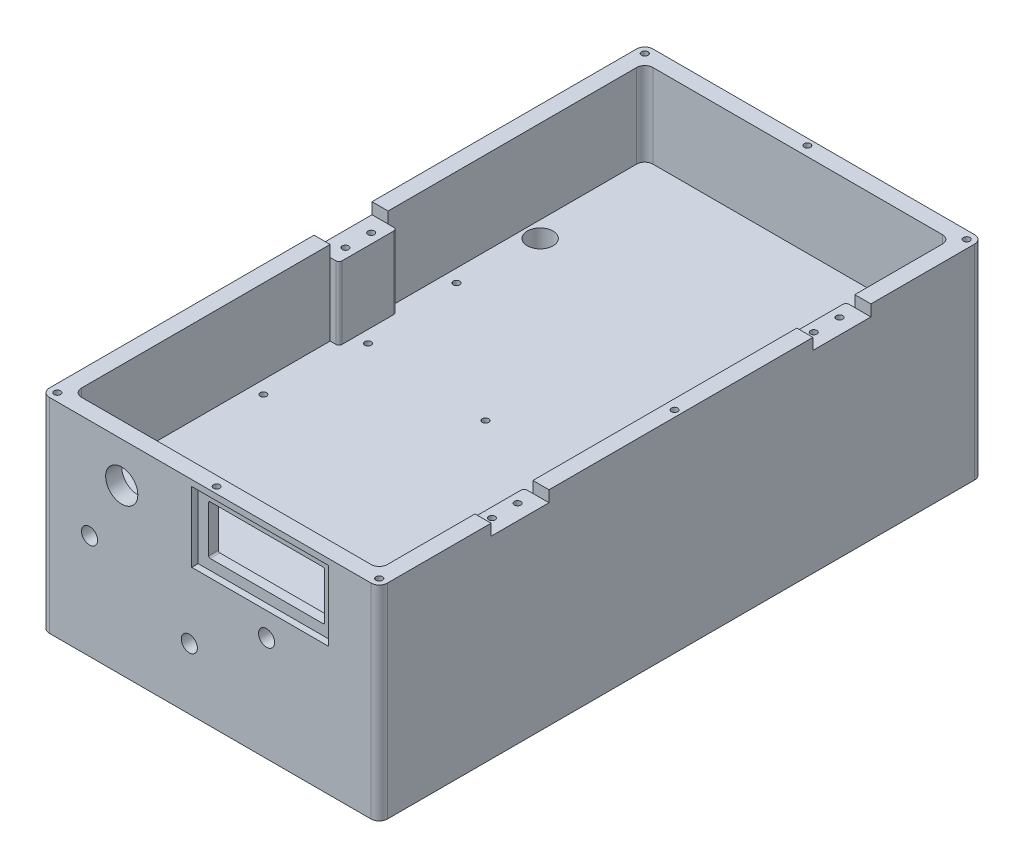
SolidWorks part; units mm, degrees
ref_plane "Front Plane" through (0, 0, 0) normal (0, 0, 1) x (1, 0, 0)
ref_plane "Top Plane" through (0, 0, 0) normal (0, 1, 0) x (1, 0, 0)
ref_plane "Right Plane" through (0, 0, 0) normal (1, 0, 0) x (0, 0, -1)
sketch "Sketch1" plane through (0, 0, 0) normal (0, 1, 0) x (1, 0, 0)
  line L1 (0, 0) -> (200, 0)
  line L2 (0, 0) -> (0, 400)
  line L3 (0, 400) -> (200, 400)
  line L4 (200, 0) -> (200, 400)
extrude "Boss-Extrude1" add sketch "Sketch1" along normal blind 25
sketch "Sketch2" plane through (0, 0, 0) normal (0, -1, 0) x (1, 0, 0)
  line L0 (0, -400) -> (0, 0) construction
  line L1 (37.7823, -177.17) -> (65.6061, -192.9762) construction
  line L2 (200, -400) -> (0, -400) construction
  line L3 (21.9762, -204.9939) -> (8.0642, -197.0908) construction
  circle A0 centre (70, -320) radius 1
  circle A1 centre (68.3, -276.5) radius 1
  circle A2 centre (66, -139.3) radius 1
  circle A3 centre (50, -320) radius 1
  circle A4 centre (50, -300) radius 1
  circle A5 centre (70, -300) radius 1
  circle A6 centre (48.3, -276.5) radius 1
  circle A7 centre (46, -139.3) radius 1
  circle A8 centre (48.3, -256.5) radius 1
  circle A9 centre (46, -119.3) radius 1
  circle A10 centre (68.3, -256.5) radius 1
  circle A11 centre (66, -119.3) radius 1
  circle A12 centre (49.8, -220.8) radius 1.5
  circle A13 centre (65.6061, -192.9762) radius 1.5
  circle A14 centre (37.7823, -177.17) radius 1.5
  circle A15 centre (21.9762, -204.9939) radius 1.5
  circle A16 centre (51.6942, -185.0731) radius 1.5
  circle A17 centre (8.0642, -197.0908) radius 1.5
  dimension "D1" = 70
  dimension "D2" = 80
  dimension "D3" = 43.5
  dimension "D4" = 1.7
  dimension "D5" = 180.7
  dimension "D6" = 4
  dimension "D11" = 99.2
  dimension "D12" = 20.2
  dimension "D7" = 2
  dimension "D8" = 2
  dimension "D9" = 2
  dimension "D10" = 2
  dimension "D13" = 2
  dimension "D14" = 2
extrude "Cut-Extrude1" cut sketch "Sketch2" against normal blind 5
sketch "Sketch3" plane through (0, 0, 0) normal (0, -1, 0) x (1, 0, 0)
  line L0 (66, -119.3) -> (46, -139.3) construction
  line L1 (56, -129.3) -> (57.9085, -144.8434) construction
  line L2 (0, -400) -> (0, 0) construction
  line L3 (57.9085, -144.8434) -> (97.891, -305.2047) construction
  line L4 (97.891, -305.2047) -> (64.0384, -102.9093) construction
  line L5 (64.0384, -102.9093) -> (134.2678, -301.231) construction
  line L6 (134.2678, -301.231) -> (118.7891, -68.1883) construction
  line L7 (118.7891, -68.1883) -> (118.7891, -348.1883) construction
  line L8 (68.3, -256.5) -> (48.3, -276.5) construction
  line L9 (58.3, -266.5) -> (60.0513, -252.2371) construction
  line L10 (60.0513, -252.2371) -> (96.3395, -106.6928) construction
  line L11 (96.3395, -106.6928) -> (82.5516, -353.3076) construction
  line L12 (82.5516, -353.3076) -> (82.5516, -73.3076) construction
  dimension "D1" = 7
  dimension "D2" = 14
  dimension "D3" = 4.5
  dimension "D4" = 10
  dimension "D5" = 15.7
  dimension "D6" = 7
  dimension "D7" = 14
  dimension "D8" = 10.8
sketch "Sketch4" plane through (0, 0, 0) normal (0, -1, 0) x (1, 0, 0)
  line L0 (97.891, -305.2047) -> (101.3054, -321.6196) construction
  line L1 (97.891, -305.2047) -> (64.0384, -102.9093) construction
  line L2 (64.0384, -102.9093) -> (59.8238, -86.6126) construction
  line L3 (64.0384, -102.9093) -> (134.2678, -301.231) construction
  line L5 (134.2678, -301.231) -> (137.9976, -319.3208) construction
  line L6 (134.2678, -301.231) -> (118.7891, -68.1883) construction
  line L7 (118.7891, -68.1883) -> (118.4009, -56.4845) construction
  line L8 (118.7891, -68.1883) -> (118.7891, -348.1883) construction
  line L9 (96.3395, -106.6928) -> (98.8592, -90.0322) construction
  line L10 (96.3395, -106.6928) -> (82.5516, -353.3076) construction
  line L11 (82.5516, -353.3076) -> (82.0812, -370.1511) construction
  line L14 (82.5516, -353.3076) -> (82.5516, -73.3076) construction
  line L16 (118.7891, -348.1883) -> (118.7891, -367.68) construction
  line L17 (82.5516, -73.3076) -> (82.5516, -58.9376) construction
  dimension "D2" = 5
  dimension "D3" = 7.85
  dimension "D4" = 1.9
  dimension "D5" = 5.4
  dimension "D6" = 1.6
  dimension "D1" = 2.25
sketch "Sketch6" plane through (0, 0, 0) normal (0, -1, 0) x (1, 0, 0)
  circle A0 centre (82, -370) radius 2
  circle A1 centre (70, -320) radius 1 construction
  circle A2 centre (59.7, -86.5) radius 2
  circle A4 centre (119.5, -370) radius 2
  circle A5 centre (82, -56.5) radius 2
  circle A6 centre (101.2, -321.7) radius 2
  circle A7 centre (138.2, -321.7) radius 2
  circle A8 centre (119, -56.5) radius 2
  circle A9 centre (99, -90) radius 2
  dimension "D1" = 50
  dimension "D2" = 12
  dimension "D3" = 37.5
  dimension "D4" = 313.5
  dimension "D5" = 12
  dimension "D6" = 48.3
  dimension "D7" = 19.2
  dimension "D8" = 37
  dimension "D9" = 37
  dimension "D10" = 17
  dimension "D11" = 33.5
  dimension "D12" = 22.3
  dimension "D13" = 30
sketch "Sketch7" plane through (0, 0, 0) normal (0, -1, 0) x (1, 0, 0)
  line L1 (200, 0) -> (-100, 0) construction
  line L2 (200, 0) -> (200, -530) construction
  line L3 (200, -530) -> (-100, -530) construction
  line L4 (-100, 0) -> (-100, -530) construction
sketch "Sketch9" plane through (0, 0, 0) normal (0, -1, 0) x (1, 0, 0)
  line L0 (75, -330) -> (90, -330)
  line L1 (50, -99) -> (200, -99)
  line L3 (110, 0) -> (200, 0)
  line L4 (200, -99) -> (200, 0)
  line L5 (200, 0) -> (200, -530) construction
  line L6 (200, -315) -> (90, -315)
  line L7 (200, -315) -> (200, -400)
  line L8 (200, -400) -> (75, -400)
  line L10 (200, -400) -> (0, -400) construction
  line L12 (75, -400) -> (40, -400)
  line L13 (40, -400) -> (40, -330)
  line L14 (40, -330) -> (75, -330)
  line L15 (90, -330) -> (90, -315)
  line L16 (50, -99) -> (50, -79)
  line L17 (50, -79) -> (100, -79)
  line L19 (100, -79) -> (110, -79)
  line L20 (110, -79) -> (110, 0)
  dimension "D1" = 85
  dimension "D3" = 35
extrude "Boss-Extrude2" add sketch "Sketch9" along normal blind 12
sketch "Sketch10" plane through (0, -12, 0) normal (0, -1, 0) x (1, 0, 0)
  circle A0 centre (82, -56.5) radius 2
  circle A1 centre (119, -56.5) radius 2
  circle A2 centre (59.7, -86.5) radius 2
  circle A3 centre (99, -90) radius 2
  circle A4 centre (138.2, -321.7) radius 2
  circle A5 centre (119.5, -370) radius 2
  circle A6 centre (101.2, -321.7) radius 2
  circle A7 centre (82, -370) radius 2
extrude "Cut-Extrude2" cut sketch "Sketch10" against normal blind 5
sketch "Sketch11" plane through (0, 25, 0) normal (0, 1, 0) x (1, 0, 0)
  line L0 (200, 400) -> (0, 400) construction
  line L1 (200, 0) -> (200, 530) construction
  line L2 (161, 200) -> (155.25, 200) construction
  line L3 (155.25, 200) -> (155.25, 273.7112) construction
  circle A0 centre (161, 200) radius 2
  circle A7 centre (91, 200) radius 2
  circle A8 centre (91, 42) radius 2
  circle A9 centre (161, 42) radius 2
  dimension "D1" = 2
  dimension "D3" = 200
  dimension "D4" = 39
  dimension "D5" = 5.75
  dimension "D2" = 2
extrude "Cut-Extrude3" cut sketch "Sketch11" against normal blind 5
sketch "Sketch13" plane through (0, 0, 0) normal (0, -1, 0) x (1, 0, 0)
  line L0 (155.25, -235) -> (155.25, -266) construction
  line L1 (165.75, -235) -> (144.75, -235)
  line L2 (165.75, -235) -> (165.75, -266)
  line L4 (144.75, -235) -> (144.75, -266)
  line L5 (200, 0) -> (200, -530) construction
  line L6 (200, 0) -> (-100, 0) construction
  line L7 (165.75, -266) -> (155.25, -266)
  line L8 (155.25, -266) -> (144.75, -266)
  dimension "D1" = 44.75
  dimension "D2" = 235
extrude "Cut-Extrude4" cut sketch "Sketch13" against normal blind 157
sketch "Sketch14" plane through (0, -12, 0) normal (0, -1, 0) x (1, 0, 0)
  line L0 (200, 0) -> (200, -530) construction
  line L1 (40, -400) -> (200, -400) construction
  line L2 (155.25, -330) -> (165.4111, -340.1611) construction
  line L3 (50, -320) -> (70, -320) construction
  line L4 (60, -320) -> (60, -330) construction
  line L5 (155.25, -330) -> (60, -330) construction
  line L6 (60, -330) -> (49.8389, -340.1611) construction
  circle A0 centre (155.25, -330) radius 2 construction
  circle A1 centre (165.4111, -340.1611) radius 2
  circle A2 centre (49.8389, -340.1611) radius 2
  dimension "D1" = 44.75
  dimension "D2" = 70
  dimension "D3" = 45
extrude "Cut-Extrude5" cut sketch "Sketch14" against normal blind 5
sketch "Sketch15" plane through (0, 0, 0) normal (0, 0, 1) x (1, 0, 0)
  line L0 (0, 25) -> (200, 25) construction
  line L1 (200, 25) -> (200, -12) construction
  circle A1 centre (130, 15) radius 3.5
  dimension "D1" = 10
  dimension "D3" = 70
extrude "Cut-Extrude6" cut sketch "Sketch15" against normal blind 175
sketch "Sketch16" plane through (0, 0, 0) normal (0, -1, 0) x (1, 0, 0)
  line L0 (200, 0) -> (200, -530) construction
  line L1 (200, 0) -> (-100, 0) construction
  line L2 (0, -400) -> (0, 0) construction
  circle A0 centre (130, -170) radius 3.5
  circle A1 centre (20, -265) radius 3.5
  dimension "D1" = 70
  dimension "D2" = 170
  dimension "D3" = 265
  dimension "D4" = 20
extrude "Cut-Extrude7" cut sketch "Sketch16" against normal blind 20
sketch "Sketch17" plane through (0, 0, 0) normal (0, 0, 1) x (1, 0, 0)
  line L0 (0, 25) -> (200, 25) construction
  line L1 (0, 25) -> (0, 0) construction
  circle A0 centre (20, 15) radius 3.5
  dimension "D1" = 10
  dimension "D2" = 20
extrude "Cut-Extrude8" cut sketch "Sketch17" against normal blind 270
sketch "Sketch18" plane through (0, 0, 0) normal (0, -1, 0) x (1, 0, 0)
  circle A0 centre (130, -170) radius 4
  circle A1 centre (20, -265) radius 4
extrude "Cut-Extrude9" cut sketch "Sketch18" against normal blind 7
sketch "Sketch19" plane through (0, 0, 0) normal (0, -1, 0) x (1, 0, 0)
  line L0 (165.75, -250.5) -> (181.25, -250.5) construction
  line L1 (165.75, -266) -> (165.75, -235) construction
  line L2 (144.75, -250.5) -> (131.25, -250.5) construction
  line L3 (144.75, -235) -> (144.75, -266) construction
  circle A0 centre (181.25, -250.5) radius 2
  circle A1 centre (131.25, -250.5) radius 2
extrude "Cut-Extrude10" cut sketch "Sketch19" against normal blind 5
sketch "Sketch20" plane through (0, -12, 0) normal (0, -1, 0) x (1, 0, 0)
  line L1 (200, 0) -> (0, 0)
  line L2 (200, 0) -> (200, -35)
  line L3 (200, -35) -> (0, -35)
  line L4 (0, 0) -> (0, -35)
extrude "Cut-Extrude11" cut sketch "Sketch20" against normal blind 98
sketch "Sketch21" plane through (0, 0, 0) normal (0, -1, 0) x (1, 0, 0)
  line L0 (82, -56.5) -> (72, -56.5) construction
  line L1 (72, -56.5) -> (72, -46.5) construction
  circle A0 centre (72, -46.5) radius 1
  circle A1 centre (92, -46.5) radius 1
  circle A2 centre (92, -66.5) radius 1
  circle A3 centre (72, -66.5) radius 1
  dimension "D1" = 2
  dimension "D2" = 2
extrude "Cut-Extrude12" cut sketch "Sketch21" against normal blind 5
sketch "Sketch22" plane through (0, -12, 0) normal (0, -1, 0) x (1, 0, 0)
  line L0 (200, 0) -> (200, -530) construction
  line L1 (40, -400) -> (200, -400) construction
  line L2 (0, -400) -> (0, -35) construction
  line L3 (0, -35) -> (110, -35) construction
  circle A0 centre (160, -370) radius 3.25
  circle A1 centre (23, -370) radius 3.25
  circle A2 centre (54, -60) radius 3.25
  dimension "D1" = 40
  dimension "D2" = 30
  dimension "D3" = 137
  dimension "D4" = 54
  dimension "D5" = 25
extrude "Cut-Extrude13" [suppressed] cut sketch "Sketch22" against normal blind 84
sketch "Sketch23" [suppressed] plane through (0, 0, 0) normal (0, -1, 0) x (1, 0, 0)
  circle A0 centre (54, -60) radius 6.25
  circle A1 centre (23, -370) radius 6.25
extrude "Cut-Extrude14" [suppressed] cut sketch "Sketch23" against normal blind 22
sketch "Sketch24" [suppressed] plane through (0, -12, 0) normal (0, -1, 0) x (1, 0, 0)
  circle A0 centre (160, -370) radius 6.25
extrude "Cut-Extrude15" [suppressed] cut sketch "Sketch24" against normal blind 34
sketch "Sketch27" plane through (0, 0, -35) normal (0, 0, 1) x (1, 0, 0)
  line L1 (0, 25) -> (200, 25)
  line L2 (0, 25) -> (0, -50)
  line L3 (0, -50) -> (200, -50)
  line L4 (200, 25) -> (200, -50)
  circle A1 centre (130, 15) radius 3.5
  circle A2 centre (20, 15) radius 3.5
extrude "Boss-Extrude3" add sketch "Sketch27" along normal blind 10
sketch "Sketch28" plane through (0, 0, -25) normal (0, 0, 1) x (1, 0, 0)
  line L0 (0, 25) -> (0, -50) construction
  line L1 (200, 25) -> (0, 25) construction
  circle A0 centre (82, -12) radius 5
  dimension "D1" = 82
  dimension "D2" = 37
extrude "Cut-Extrude16" cut sketch "Sketch28" against normal blind 10
sketch "Sketch29" plane through (0, 0, 0) normal (0, -1, 0) x (1, 0, 0)
  circle A2 centre (103, -59.5) radius 1.5
  circle A3 centre (92, -66.5) radius 1 construction
  circle A4 centre (103, -63.5) radius 1.5
  dimension "D1" = 4
  dimension "D2" = 11
  dimension "D3" = 7
extrude "Cut-Extrude17" cut sketch "Sketch29" against normal blind 5
sketch "Sketch30" plane through (0, 0, 0) normal (-1, 0, 0) x (0, 0, 1)
  line L1 (-25, 25) -> (-400, 25)
  line L2 (-25, 25) -> (-25, -50)
  line L3 (-25, -50) -> (-400, -50)
  line L4 (-400, 25) -> (-400, -50)
extrude "Boss-Extrude4" add sketch "Sketch30" along normal blind 10
sketch "Sketch31" plane through (0, 0, -400) normal (0, 0, -1) x (-1, 0, 0)
  line L1 (10, -50) -> (-200, -50)
  line L2 (10, -50) -> (10, 25)
  line L3 (10, 25) -> (-200, 25)
  line L4 (-200, -50) -> (-200, 25)
extrude "Boss-Extrude5" add sketch "Sketch31" against normal blind 10
sketch "Sketch32" plane through (200, 0, 0) normal (1, 0, 0) x (0, 0, -1)
  line L1 (400, -50) -> (25, -50)
  line L2 (400, -50) -> (400, 25)
  line L3 (400, 25) -> (25, 25)
  line L4 (25, -50) -> (25, 25)
extrude "Boss-Extrude6" add sketch "Sketch32" against normal blind 10
sketch "Sketch33" plane through (0, -12, 0) normal (0, -1, 0) x (1, 0, 0)
  line L0 (190, -390) -> (0, -390) construction
  line L1 (40, -330) -> (40, -390) construction
  circle A0 centre (95, -341) radius 1.5
  circle A1 centre (140, -341) radius 1.5
  dimension "D1" = 49
  dimension "D2" = 55
  dimension "D3" = 45
extrude "Cut-Extrude18" cut sketch "Sketch33" against normal blind 5
sketch "Sketch34" plane through (0, 25, 0) normal (0, 1, 0) x (1, 0, 0)
  line L1 (200, 400) -> (-10, 400)
  line L2 (200, 400) -> (200, 25)
  line L3 (200, 25) -> (-10, 25)
  line L4 (-10, 400) -> (-10, 25)
  line L5 (190, 390) -> (190, 35)
  line L6 (190, 35) -> (0, 35)
  line L7 (0, 35) -> (0, 390)
  line L8 (0, 390) -> (190, 390)
extrude "Boss-Extrude7" add sketch "Sketch34" along normal blind 52
sketch "Sketch35" plane through (0, 0, -25) normal (0, 0, 1) x (1, 0, 0)
  line L0 (-10, -50) -> (200, -50) construction
  line L1 (167, 70) -> (87, 70)
  line L2 (167, 70) -> (167, 40)
  line L3 (167, 40) -> (87, 40)
  line L4 (87, 70) -> (87, 40)
  line L5 (200, -50) -> (200, 77) construction
  dimension "D1" = 30
  dimension "D2" = 80
  dimension "D3" = 90
  dimension "D4" = 33
extrude "Cut-Extrude19" cut sketch "Sketch35" against normal blind 35
sketch "Sketch36" plane through (0, -50, 0) normal (0, -1, 0) x (1, 0, 0)
  line L0 (0, -390) -> (0, -35) construction
  line L1 (-3, -391) -> (-1, -391)
  line L2 (-3, -391) -> (-3, -34)
  line L3 (-3, -34) -> (-1, -34)
  line L4 (-1, -391) -> (-1, -34)
  line L5 (190, -390) -> (0, -390) construction
  line L6 (0, -35) -> (190, -35) construction
  line L7 (95, -400) -> (95, -25) construction
  line L8 (-10, -400) -> (200, -400) construction
  line L9 (-10, -25) -> (200, -25) construction
  line L10 (191, -391) -> (191, -34)
  line L11 (193, -34) -> (191, -34)
  line L12 (193, -391) -> (193, -34)
  line L13 (193, -391) -> (191, -391)
  dimension "D1" = 2
  dimension "D2" = 1
  dimension "D3" = 1
  dimension "D4" = 1
extrude "Cut-Extrude20" cut sketch "Sketch36" against normal blind 1.5
sketch "Sketch37" plane through (0, -50, 0) normal (0, -1, 0) x (1, 0, 0)
  line L1 (-3, -391) -> (193, -391)
  line L2 (-3, -391) -> (-3, -393)
  line L3 (-3, -393) -> (193, -393)
  line L4 (193, -391) -> (193, -393)
  line L5 (-3, -34) -> (193, -34)
  line L6 (-3, -34) -> (-3, -32)
  line L7 (-3, -32) -> (193, -32)
  line L8 (193, -34) -> (193, -32)
extrude "Cut-Extrude21" cut sketch "Sketch37" against normal blind 1.5
sketch "Sketch38" plane through (0, -50, 0) normal (0, -1, 0) x (1, 0, 0)
  line L0 (-10, -25) -> (200, -25) construction
  line L1 (193, -393) -> (193, -32) construction
  line L4 (95, -400) -> (95, -25) construction
  line L5 (-10, -400) -> (200, -400) construction
  line L6 (-10, -212.5) -> (200, -212.5) construction
  line L7 (-10, -400) -> (-10, -25) construction
  line L8 (200, 0) -> (200, -530) construction
  circle A1 centre (195, -30) radius 2
  circle A5 centre (95, -396) radius 2
  circle A6 centre (95, -29) radius 2
  circle A7 centre (-6, -212.5) radius 2
  circle A8 centre (196, -212.5) radius 2
  circle A9 centre (-5, -30) radius 2
  circle A10 centre (-5, -395) radius 2
  circle A11 centre (195, -395) radius 2
  dimension "D1" = 5
  dimension "D2" = 2
  dimension "D3" = 2
  dimension "D4" = 2
extrude "Cut-Extrude22" cut sketch "Sketch38" against normal blind 5
fillet "Fillet1" radius 5 4 edges at (200, 13.5, -25) (-10, 13.5, -25) (200, 13.5, -400) (-10, 13.5, -400)
fillet "Fillet4" radius 5 4 edges at (190, -31, -35) (0, -25, -35) (0, -25, -390) (190, -31, -390)
fillet "Fillet5" radius 5 8 edges at (-1, -49.25, -34) (-3, -49.25, -32) (191, -49.25, -34) (193, -49.25, -32) (193, -49.25, -393) (191, -49.25, -391) (-1, -49.25, -391) (-3, -49.25, -393)
fillet "Fillet6" radius 5 4 edges at (0, 51, -35) (190, 51, -35) (0, 51, -390) (190, 51, -390)
sketch "Sketch41" plane through (0, 0, -400) normal (0, 0, -1) x (-1, 0, 0)
  line L0 (-200, -50) -> (-200, 77) construction
  line L1 (5, -50) -> (-195, -50) construction
  circle A0 centre (-119.5, -24.7) radius 5
  dimension "D1" = 80.5
  dimension "D2" = 25.3
extrude "Cut-Extrude23" cut sketch "Sketch41" against normal blind 28
sketch "Sketch42" plane through (0, -12, 0) normal (0, -1, 0) x (1, 0, 0)
  line L0 (-5, -400) -> (195, -400) construction
  line L1 (200, 0) -> (200, -530) construction
  circle A0 centre (155, -375) radius 2
  dimension "D1" = 25
  dimension "D2" = 45
extrude "Cut-Extrude24" cut sketch "Sketch42" against normal blind 5
sketch "Sketch43" plane through (0, 0, 0) normal (0, -1, 0) x (1, 0, 0)
  line L0 (-10, -395) -> (-10, -30) construction
  line L1 (-5, -400) -> (195, -400) construction
  circle A0 centre (10, -385) radius 2
  circle A1 centre (10, -364) radius 2
  dimension "D1" = 21
  dimension "D2" = 20
  dimension "D3" = 15
extrude "Cut-Extrude25" cut sketch "Sketch43" against normal blind 5
sketch "Sketch44" plane through (0, 0, 0) normal (0, -1, 0) x (1, 0, 0)
  line L0 (-5, -400) -> (195, -400) construction
  line L1 (-10, -395) -> (-10, -30) construction
  circle A0 centre (10, -315) radius 8
  dimension "D1" = 85
  dimension "D2" = 20
extrude "Cut-Extrude26" cut sketch "Sketch44" against normal blind 59
sketch "Sketch45" plane through (0, 25, 0) normal (0, 1, 0) x (1, 0, 0)
  line L0 (0, 385) -> (0, 40) construction
  circle A0 centre (8, 265) radius 2
  circle A1 centre (8, 205) radius 2 construction
  circle A2 centre (8, 145) radius 2
  circle A3 centre (8, 85) radius 2
  circle A4 centre (13, 205) radius 2
  dimension "D1" = 8
  dimension "D2" = 240
  dimension "D3" = 60
  dimension "D5" = 5
  dimension "D4" = 3
extrude "Cut-Extrude27" cut sketch "Sketch45" against normal blind 5
sketch "Sketch46" plane through (0, 0, -25) normal (0, 0, 1) x (1, 0, 0)
  line L0 (-5, 77) -> (195, 77) construction
  line L1 (-10, -50) -> (-10, 77) construction
  circle A0 centre (40, 52) radius 10
  dimension "D1" = 25
  dimension "D2" = 50
extrude "Cut-Extrude28" cut sketch "Sketch46" against normal blind 42
sketch "Sketch47" plane through (0, 0, -25) normal (0, 0, 1) x (1, 0, 0)
  circle A0 centre (20, 15) radius 5
  circle A1 centre (130, 15) radius 5
extrude "Cut-Extrude29" cut sketch "Sketch47" against normal blind 20
sketch "Sketch48" plane through (0, 77, 0) normal (0, 1, 0) x (1, 0, 0)
  line L0 (195, 400) -> (-5, 400) construction
  line L1 (-17.5, 400.3951) -> (-17.5, 19.7403) construction
  line L3 (200, 0) -> (200, 530) construction
  line L4 (0, 212.5) -> (190, 212.5) construction
  line L5 (0, 385) -> (0, 40) construction
  line L6 (190, 40) -> (190, 385) construction
  line L8 (-10, 395) -> (-10, 30) construction
  line L9 (207.5, 400.3951) -> (207.5, 25.2099) construction
  circle A0 centre (-0.5, 220.5) radius 3
  circle A1 centre (-0.5, 204.5) radius 3
  circle A4 centre (190.5, 320.5) radius 3
  circle A5 centre (190.5, 304.5) radius 3
  circle A6 centre (190.5, 120.5) radius 3
  circle A7 centre (190.5, 104.5) radius 3
  dimension "D1" = 16
  dimension "D2" = 179.5
  dimension "D3" = 9.5
  dimension "D4" = 16
  dimension "D6" = 92
  dimension "D7" = 9.5
  dimension "D8" = 9.5
  dimension "D5" = 17
  dimension "D9" = 17
sketch "Sketch49" plane through (0, 77, 0) normal (0, 1, 0) x (1, 0, 0)
  line L0 (0, 212.5) -> (0, 230.5)
  line L1 (0, 385) -> (0, 40) construction
  line L2 (0, 230.5) -> (5.5, 230.5)
  line L3 (5.5, 230.5) -> (5.5, 194.5)
  line L4 (5.5, 194.5) -> (0, 194.5)
  line L5 (0, 385) -> (0, 40) construction
  line L6 (0, 194.5) -> (0, 212.5)
  line L7 (190.5, 320.5) -> (190.5, 304.5) construction
  line L8 (0, 212.5) -> (190, 212.5) construction
  line L9 (190, 312.5) -> (190, 330.5)
  line L10 (190, 40) -> (190, 385) construction
  line L11 (190, 330.5) -> (184.5, 330.5)
  line L12 (184.5, 330.5) -> (184.5, 294.5)
  line L13 (184.5, 294.5) -> (190, 294.5)
  line L14 (190, 294.5) -> (190, 312.5)
  line L15 (190.5, 104.5) -> (190.5, 120.5) construction
  line L16 (190, 130.5) -> (190, 112.5)
  line L17 (184.5, 130.5) -> (190, 130.5)
  line L18 (184.5, 94.5) -> (184.5, 130.5)
  line L19 (190, 94.5) -> (184.5, 94.5)
  line L20 (190, 112.5) -> (190, 94.5)
  circle A0 centre (190.5, 320.5) radius 3 construction
  dimension "D1" = 18
  dimension "D2" = 18
  dimension "D3" = 10
extrude "Boss-Extrude8" add sketch "Sketch49" against normal blind 52
sketch "Sketch51" plane through (0, 77, 0) normal (0, 1, 0) x (1, 0, 0)
  line L5 (200, 0) -> (200, 530) construction
  line L6 (184.5, 330.5) -> (200, 330.5)
  line L7 (184.5, 330.5) -> (184.5, 294.5)
  line L8 (184.5, 294.5) -> (200, 294.5)
  line L9 (200, 330.5) -> (200, 294.5)
  line L10 (-10, 395) -> (-10, 30) construction
  line L11 (184.5, 130.5) -> (200, 130.5)
  line L12 (184.5, 130.5) -> (184.5, 94.5)
  line L13 (184.5, 94.5) -> (200, 94.5)
  line L14 (200, 130.5) -> (200, 94.5)
  line L15 (5.5, 194.5) -> (-10, 194.5)
  line L16 (5.5, 194.5) -> (5.5, 230.5)
  line L17 (5.5, 230.5) -> (-10, 230.5)
  line L18 (-10, 194.5) -> (-10, 230.5)
extrude "Cut-Extrude31" cut sketch "Sketch51" against normal blind 7
sketch "Sketch52" plane through (0, 70, 0) normal (0, 1, 0) x (1, 0, 0)
  circle A0 centre (-0.5, 220.5) radius 2
  circle A1 centre (-0.5, 204.5) radius 2
  circle A2 centre (190.5, 104.5) radius 2
  circle A3 centre (190.5, 120.5) radius 2
  circle A4 centre (190.5, 320.5) radius 2
  circle A5 centre (190.5, 304.5) radius 2
extrude "Cut-Extrude32" cut sketch "Sketch52" against normal blind 5
fillet "Fillet7" radius 2 6 edges at (184.5, 47.5, -94.5) (184.5, 47.5, -130.5) (184.5, 47.5, -294.5) (184.5, 47.5, -330.5) (5.5, 47.5, -194.5) (5.5, 47.5, -230.5)
sketch "Sketch53" plane through (0, 77, 0) normal (0, 1, 0) x (1, 0, 0)
  circle A0 centre (-5, 30) radius 2
  circle A1 centre (95, 29) radius 2
  circle A2 centre (195, 30) radius 2
  circle A3 centre (196, 212.5) radius 2
  circle A4 centre (195, 395) radius 2
  circle A5 centre (95, 396) radius 2
  circle A6 centre (-5, 395) radius 2
extrude "Cut-Extrude33" cut sketch "Sketch53" against normal blind 5
sketch "Sketch55" plane through (0, 25, 0) normal (0, 1, 0) x (1, 0, 0)
  line L0 (155.25, 266) -> (155.25, 235) construction
  line L1 (144.75, 266) -> (165.75, 266) construction
  line L2 (165.75, 235) -> (144.75, 235) construction
  line L3 (165.75, 250.5) -> (144.75, 250.5) construction
  line L4 (165.75, 266) -> (165.75, 235) construction
  line L5 (144.75, 235) -> (144.75, 266) construction
  circle A0 centre (161.25, 269.5) radius 1.5
  circle A1 centre (149.25, 269.5) radius 1.5
  circle A2 centre (149.25, 231.5) radius 1.5
  circle A3 centre (161.25, 231.5) radius 1.5
  dimension "D1" = 19
  dimension "D2" = 6
  dimension "D3" = 6
sketch "Sketch56" plane through (0, 0, 0) normal (0, -1, 0) x (1, 0, 0)
  circle A0 centre (161.25, -231.5) radius 1.5
  circle A1 centre (149.25, -231.5) radius 1.5
  circle A2 centre (161.25, -269.5) radius 1.5
  circle A3 centre (149.25, -269.5) radius 1.5
extrude "Cut-Extrude35" cut sketch "Sketch56" against normal blind 5
other "Move Face1" face at (167, 55, -30) parameters "D1"=5
other "Move Face2" face at (87, 55, -30) parameters "D1"=3
other "Move Face3" face at (126, 40, -30) parameters "D1"=3.75
other "Move Face4" face at (126, 70, -30) parameters "D1"=3.25
sketch "Sketch57" plane through (0, 0, -25) normal (0, 0, 1) x (1, 0, 0)
  line L0 (162, 36.25) -> (162, 66.75) construction
  line L3 (90, 66.75) -> (90, 36.25) construction
  line L6 (90, 36.25) -> (162, 36.25) construction
  line L7 (83.5, 73.25) -> (168.5, 73.25)
  line L8 (83.5, 73.25) -> (83.5, 29.75)
  line L9 (83.5, 29.75) -> (168.5, 29.75)
  line L10 (168.5, 73.25) -> (168.5, 29.75)
  line L11 (162, 66.75) -> (90, 66.75) construction
  dimension "D1" = 6.5
  dimension "D2" = 6.5
  dimension "D3" = 6.5
  dimension "D4" = 6.5
extrude "Cut-Extrude36" cut sketch "Sketch57" against normal blind 4
sketch "Sketch60" [suppressed] plane through (0, 0, -25) normal (0, 0, 1) x (1, 0, 0)
  line L0 (169.5, 37.25) -> (169.5, 72.75)
  line L1 (169.5, 72.75) -> (94.185, 72.75)
  line L2 (163.25, 39.5) -> (163.25, 40) construction
  line L3 (163.25, 70.5) -> (90.75, 70.5) construction
  line L4 (90.75, 39.5) -> (163.25, 39.5) construction
  line L5 (84.5, 37.25) -> (84.5, 72.75)
  line L6 (90.75, 70.5) -> (90.75, 70) construction
  line L7 (169.5, 37.25) -> (84.5, 37.25)
  line L8 (94.185, 72.75) -> (84.5, 72.75)
  dimension "D1" = 6.25
  dimension "D2" = 2.25
  dimension "D3" = 2.25
  dimension "D4" = 6.25
extrude "Cut-Extrude39" [suppressed] cut sketch "Sketch60" against normal blind 3
fillet "Fillet8" radius 1 4 edges at (162, 66.75, -32) (90, 66.75, -32) (90, 36.25, -32) (162, 36.25, -32)
